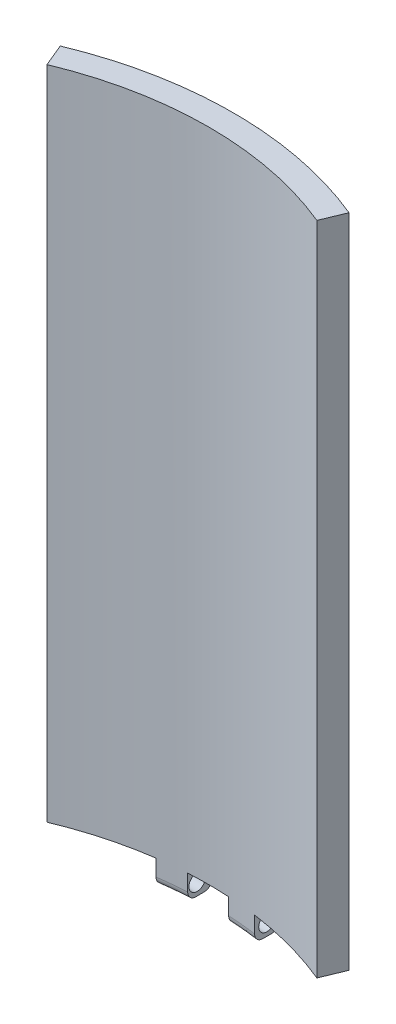
from build123d import *

# Parameters (mm, degrees)
EXTRUDE_1_DEPTH     = 3
SKETCH_7_R          = 1
CUT_EXTRUDE_2_DEPTH = 6.5
FILLET_3_R          = 1
CUT_EXTRUDE_START   = -43.5
SKETCH_8_R          = 1.5
CUT_EXTRUDE_3_DEPTH = 51.446160402


with BuildPart() as part:
    # 草图4 for 放样1 → 放样1 section 0
    with BuildSketch(Plane(origin=(0, 80, 0), x_dir=(1, 0, 0), z_dir=(0, 1, 0))):
        with BuildLine():
            Line((-17.603437889, 42.498458496), (-16.455387592, 39.726819898))
            # circular arc as an exact rational Bezier (weights 1, cos(half-angle), 1)
            Bezier((-16.455387592, 39.726819898), (0, 46.542864613), (16.455387592, 39.726819898), weights=[1, 0.923879533, 1])
            Line((16.455387592, 39.726819898), (17.603437889, 42.498458496))
            Bezier((17.603437889, 42.498458496), (0, 49.790041213), (-17.603437889, 42.498458496), weights=[1, 0.923879533, 1])
        make_face()
    # 草图3 for 放样1 → 放样1 section 1
    with BuildSketch(Plane(origin=(0, 0, 0), x_dir=(1, 0, 0), z_dir=(0, 1, 0))):
        with BuildLine():
            Line((-17.603437889, 42.498458496), (-16.455387592, 39.726819898))
            Bezier((-16.455387592, 39.726819898), (0, 46.542864613), (16.455387592, 39.726819898), weights=[1, 0.923879533, 1])
            Line((16.455387592, 39.726819898), (17.603437889, 42.498458496))
            Bezier((17.603437889, 42.498458496), (0, 49.790041213), (-17.603437889, 42.498458496), weights=[1, 0.923879533, 1])
        make_face()
    loft()

    # 草图6 → 凸台-拉伸1 (add)
    with BuildSketch(Plane.XZ):
        with BuildLine():
            Line((-6.009200316, -42.57804025), (-6.009200316, -45.605805678))
            ThreePointArc((-6.009200316, -45.605805678), (-4.257725406, -45.802530218), (-2.5, -45.932014979))
            Line((-2.5, -45.932014979), (-2.5, -42.927264064))
            ThreePointArc((-2.5, -42.927264064), (-4.258181751, -42.788642046), (-6.009200316, -42.57804025))
        make_face()
        with BuildLine():
            ThreePointArc((2.5, -45.932014979), (4.257725406, -45.802530218), (6.009200316, -45.605805678))
            Line((6.009200316, -45.605805678), (6.009200316, -42.57804025))
            ThreePointArc((6.009200316, -42.57804025), (4.258181751, -42.788642046), (2.5, -42.927264064))
            Line((2.5, -42.927264064), (2.5, -45.932014979))
        make_face()
    extrude(amount=EXTRUDE_1_DEPTH)

    # 草图7 → 切除-拉伸2 (cut, symmetric)
    with BuildSketch(Plane(origin=(0, 0, 0), x_dir=(0, 0, -1), z_dir=(1, 0, 0))):
        with Locations((44.081332421, -1.518353576)):
            Circle(SKETCH_7_R)
    extrude(amount=CUT_EXTRUDE_2_DEPTH, both=True, mode=Mode.SUBTRACT)

    # 圆角3
    fillet_3_edges = [part.edges().sort_by_distance(p)[0] for p in [
        (4.257725406, -3, -45.802530218),
        (4.258181751, -3, -42.788642046),
        (-4.257725406, -3, -45.802530218),
        (-4.258181751, -3, -42.788642046),
    ]]
    fillet(fillet_3_edges, radius=FILLET_3_R)

    # 草图8 → 切除-拉伸3 (cut, through all)
    with BuildSketch(Plane.XY.offset(CUT_EXTRUDE_START)):
        with Locations((0, 40)):
            Circle(SKETCH_8_R)
    extrude(amount=-CUT_EXTRUDE_3_DEPTH, mode=Mode.SUBTRACT)


solid = part.part
